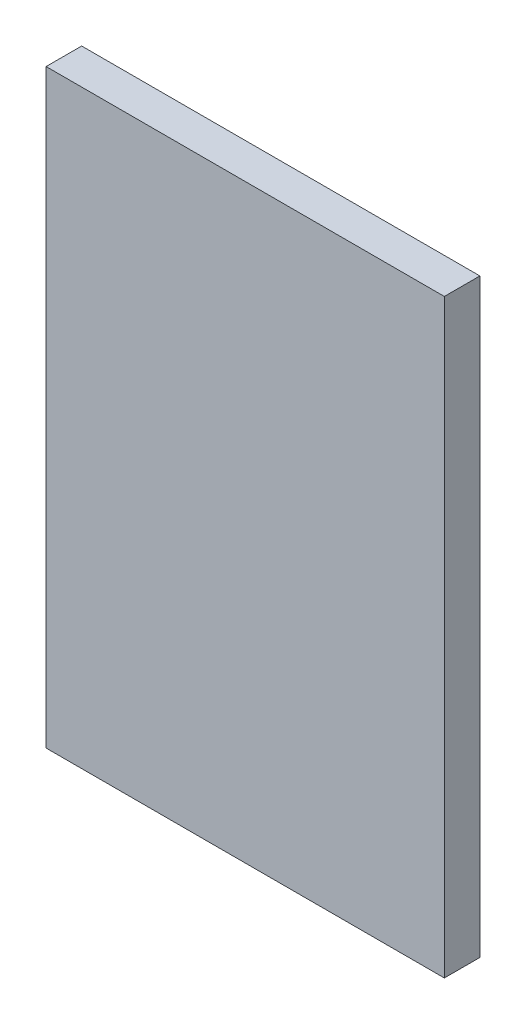
SolidWorks part; units mm, degrees
ref_plane "Front Plane" through (0, 0, 0) normal (0, 0, 1) x (1, 0, 0)
ref_plane "Top Plane" through (0, 0, 0) normal (0, 1, 0) x (1, 0, 0)
ref_plane "Right Plane" through (0, 0, 0) normal (1, 0, 0) x (0, 0, -1)
sketch "Sketch1" plane through (0, 0, 0) normal (0, 0, 1) x (1, 0, 0)
  line L6 (-140, 207.5) -> (140, 207.5)
  line L8 (-140, 207.5) -> (-140, -207.5)
  line L16 (-140, -207.5) -> (140, -207.5)
  line L17 (140, 207.5) -> (140, -207.5)
  line L18 (-140, 207.5) -> (140, -207.5) construction
  line L19 (-140, -207.5) -> (140, 207.5) construction
  point P0 (0, 0)
  point P1 (0, 0)
  point P13 (0, -332.5)
  dimension "D1" = 280
  dimension "D2" = 415
extrude "Boss-Extrude1" add sketch "Sketch1" along normal blind 25
